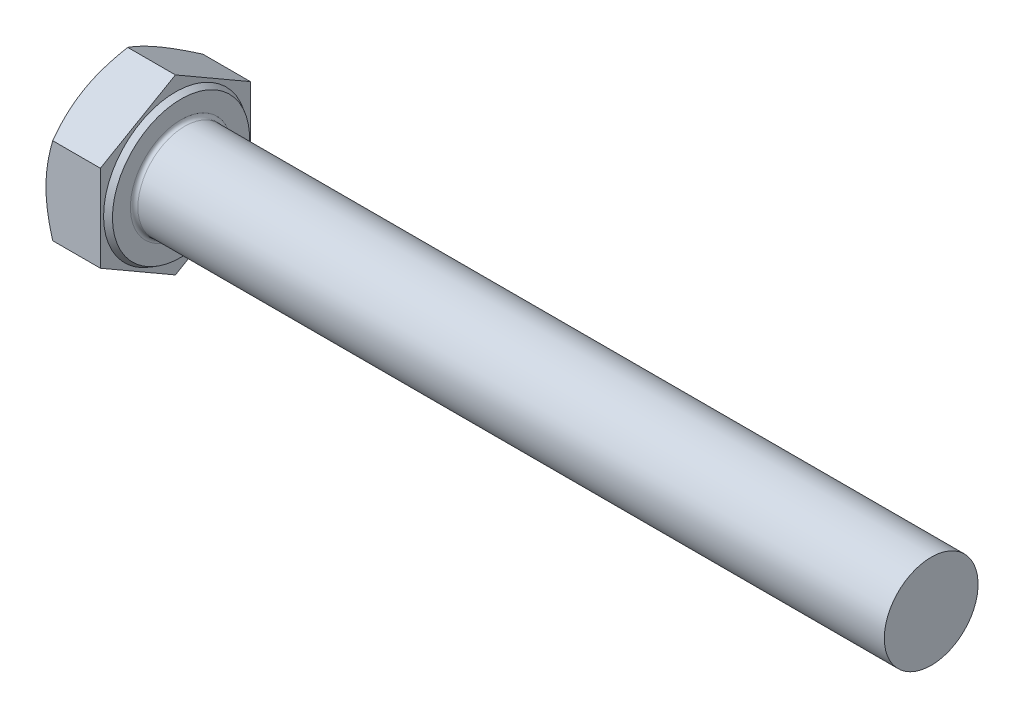
SolidWorks part; units mm, degrees
ref_plane "前视" through (0, 0, 0) normal (0, 0, 1) x (1, 0, 0)
ref_plane "上视" through (0, 0, 0) normal (0, 1, 0) x (1, 0, 0)
ref_plane "右视" through (0, 0, 0) normal (1, 0, 0) x (0, 0, -1)
sketch "草图1" plane through (0, 0, 0) normal (1, 0, 0) x (0, 0, -1)
  line L0 (8, 4.6188) -> (8, -4.6188)
  line L1 (-8, 4.6188) -> (-8, -4.6188)
  line L2 (8, -4.6188) -> (0, -9.2376)
  line L3 (0, -9.2376) -> (-8, -4.6188)
  line L4 (8, 4.6188) -> (0, 9.2376)
  line L5 (0, 9.2376) -> (-8, 4.6188)
  circle A0 centre (0, 0) radius 8.885 construction
  dimension "e" = 17.77
  dimension "s" = 16
  dimension "D2" = 120
  dimension "D3" = 8
  dimension "D4" = 8
  dimension "D5" = 8
extrude "基体-拉伸" add sketch "草图1" along normal blind 6.4
sketch "草图2" plane through (0, 0, 0) normal (0, 0, 1) x (1, 0, 0)
  line L0 (0, 4.6188) -> (0, -4.6188) construction
  line L1 (0, 0) -> (86.4, 0)
  line L2 (0, 0) -> (0, 5)
  line L3 (0, 5) -> (60.4, 5)
  line L4 (86.4, 0) -> (86.4, 3.701)
  line L5 (6.4, 9.2376) -> (6.4, 4.6188) construction
  line L7 (0, 0) -> (96.4, 0) construction
  line L8 (86.4, -3.701) -> (60.4, -5) construction
  line L9 (0, -5) -> (60.4, -5) construction
  line L10 (7.9, 5) -> (7.9, 0) construction
  line L11 (60.4, 15.24) -> (60.4, -1.27) construction
  line L12 (6.4, 4.6188) -> (6.4, -4.6188) construction
  line L13 (60.4, 5) -> (86.4, 5)
  line L14 (86.4, 5) -> (86.4, 3.701)
  dimension "l" = 80
  dimension "d" = 10
  dimension "Minor_dia" = 7.402
  dimension "p" = 1.5
  dimension "b" = 26
  dimension "ds" = 10
revolve "凸台-旋转1" add sketch "草图2" angle 360 about L7
cosmetic thread "螺旋线1" parameters "Thread_length"=26, "Thread_minor"=7.402
sketch "草图3" plane through (0, 0, 0) normal (0, 0, 1) x (1, 0, 0)
  line L0 (0, 8) -> (3.6013, 14.2376)
  line L1 (0, 9.2376) -> (0, 4.6188) construction
  line L2 (3.6013, 14.2376) -> (3.6013, 19.2376)
  line L3 (3.6013, 19.2376) -> (-10, 19.2376)
  line L4 (-10, 19.2376) -> (-10, 8)
  line L5 (-10, 8) -> (0, 8)
  line L6 (0, 0) -> (99.06, 0) construction
  line L7 (6.4, 9.2376) -> (0, 9.2376) construction
  dimension "D1" = 8
  dimension "D2" = 5
  dimension "D3" = 10
  dimension "D4" = 5
  dimension "Head_ch_ang" = 30
revolve "切除-旋转1" cut sketch "草图3" angle 360 about L6
sketch "草图4" plane through (0, 0, 0) normal (0, 0, 1) x (1, 0, 0)
  line L0 (6.4, 0) -> (6.4, 7.315) construction
  line L2 (6.4, -5) -> (6.4, 5) construction
  line L3 (6.4, 9.2376) -> (6.4, 4.6188) construction
  line L4 (6.4, 7.315) -> (5.8, 7.6614)
  line L5 (0, 0) -> (95.25, 0) construction
  line L6 (0, 0) -> (96.4, 0) construction
  line L9 (5.8, 7.6614) -> (5.8, 9.2376)
  line L10 (6.4, 9.2376) -> (0.7145, 9.2376) construction
  line L11 (5.8, 9.2376) -> (6.4, 9.2376)
  line L12 (6.4, 9.2376) -> (6.4, 7.315)
  dimension "D1" = 120
  dimension "c" = 0.6
  dimension "dw" = 14.63
revolve "切除-旋转3" cut sketch "草图4" angle 360 about L5
fillet "圆角" radius 0.4 1 edges at (6.4, 0, -5)
sketch "草图6" plane through (0, 0, 0) normal (0, 0, 1) x (1, 0, 0)
  line L0 (0, 0) -> (86.4, 0) construction
  line L1 (86.4, -5) -> (86.4, 5) construction
  line L2 (86.4, 0) -> (86.4, 5) construction
  line L4 (85.65, 5) -> (87.15, 5)
  line L5 (85.65, 5) -> (86.4, 3.701)
  line L6 (86.4, 3.701) -> (87.15, 5)
  dimension "D1" = 1.5
revolve "切除-旋转4" [suppressed] cut sketch "草图6" angle 360 about L0
pattern_linear "阵列(线性)1" [suppressed]
